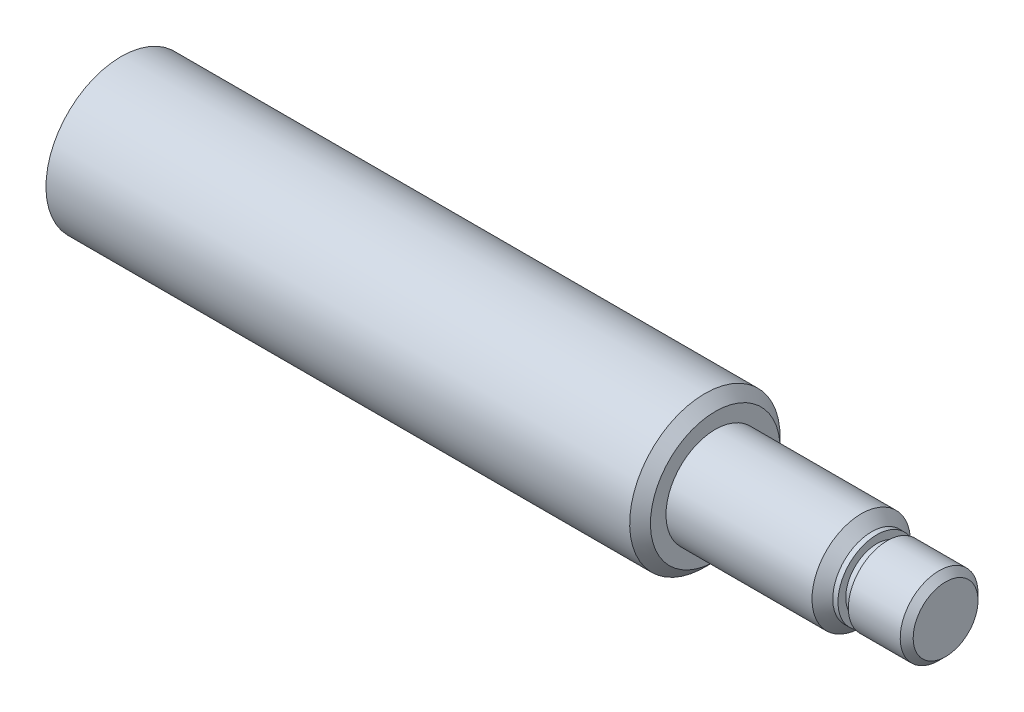
from build123d import *


with BuildPart() as part:
    # Sketch1 → Revolve1 (revolve)
    with BuildSketch(Plane.XY):
        Polygon((828.372635386, 15), (808.372635386, 15), (808.372635386, 12), (804.372635386, 12), (804.372635386, 15), (802.372635386, 15), (798.372635386, 19), (742.072635386, 19), (742.072635386, 25), (738.072635386, 29), (684.582635386, 29), (666.582635386, 29), (513.022635386, 29), (513.022635386, 0), (830.872635386, 0), (830.872635386, 12.5), align=None)
    revolve(axis=Axis((838.372635386, 0, 0), (-1, 0, 0)))


solid = part.part
